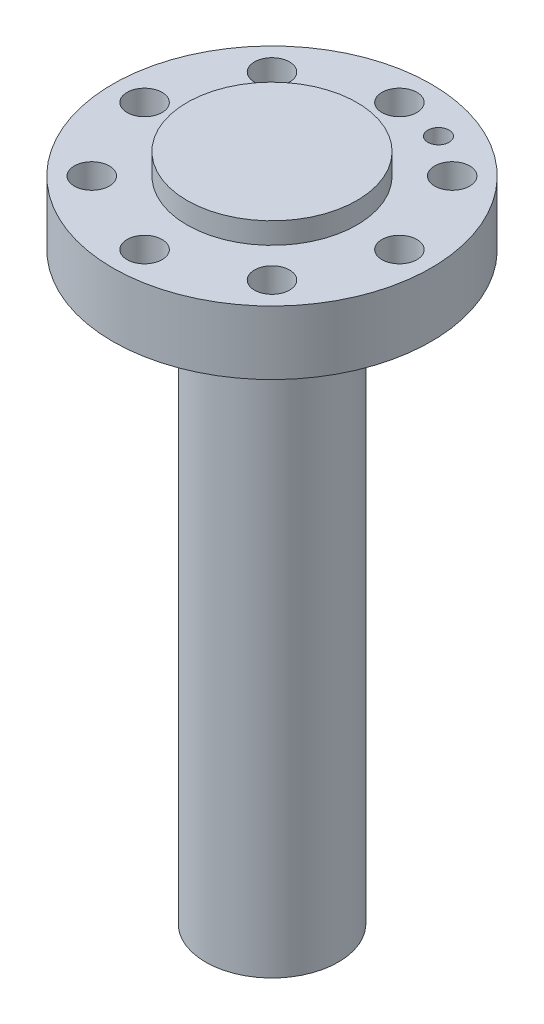
from build123d import *

# Parameters (mm, degrees)
SKETCH_1_R               = 30
EXTRUDE_1_DEPTH          = 122
CUT_EXTRUDE_START        = -12
SKETCH_2_OUTSIDE_W       = 91.722
SKETCH_2_OUTSIDE_H       = 91.722
SKETCH_2_OUTSIDE_R       = 12.5
CUT_EXTRUDE_1_DEPTH      = 118.16655914
HOLE_WIZARD_M6_1_D       = 6.6
SKETCH_7_R               = 16
EXTRUDE_3_DEPTH          = 4
MM_0_D                   = 4
HOLE_WIZARD_M6_1_2_D     = 5
HOLE_WIZARD_M6_1_2_DEPTH = 15
HOLE_WIZARD_M6_1_2_TIP   = 1.502151548


with BuildPart() as part:
    # 草图1 → 凸台-拉伸1 (new body)
    with BuildSketch(Plane(origin=(0, 0, 0), x_dir=(1, 0, 0), z_dir=(0, 1, 0))):
        with Locations(Location((0, 0, 0), (0, 0, 90))):
            Circle(SKETCH_1_R)
    extrude(amount=EXTRUDE_1_DEPTH)

    # 草图2 outside → 切除-拉伸1 (cut, through all)
    with BuildSketch(Plane(origin=(0, 122, 0), x_dir=(1, 0, 0), z_dir=(0, 1, 0)).offset(CUT_EXTRUDE_START)):
        Rectangle(SKETCH_2_OUTSIDE_W, SKETCH_2_OUTSIDE_H)
        with Locations(Location((0, 0, 0), (0, 0, 270))):
            Circle(SKETCH_2_OUTSIDE_R, mode=Mode.SUBTRACT)
    extrude(amount=-CUT_EXTRUDE_1_DEPTH, mode=Mode.SUBTRACT)

    # Hole Wizard M6 _1 (through all)
    with Locations(Plane(origin=(0, 110, 0), x_dir=(-1, 0, 0), z_dir=(0, -1, 0))):
        with Locations((-24, 0), (-16.970562748, 16.970562748), (0, 24), (16.970562748, 16.970562748), (24, 0), (16.970562748, -16.970562748), (0, -24), (-16.970562748, -16.970562748)):
            Hole(HOLE_WIZARD_M6_1_D / 2)

    # 草图7 → 凸台-拉伸3 (add)
    with BuildSketch(Plane(origin=(0, 122, 0), x_dir=(1, 0, 0), z_dir=(0, 1, 0))):
        with Locations(Location((0, 0, 0), (0, 0, 270))):
            Circle(SKETCH_7_R)
    extrude(amount=EXTRUDE_3_DEPTH)

    # 大小mm 暗销孔0 (through all)
    with Locations(Plane(origin=(0, 110, 0), x_dir=(-1, 0, 0), z_dir=(0, -1, 0))):
        with Locations((-9.184402377, 22.17310878)):
            Hole(MM_0_D / 2)

    # Hole Wizard M6 _1 2
    with Locations(Plane(origin=(0, 0, 0), x_dir=(-1, 0, 0), z_dir=(0, -1, 0))):
        with Locations((0, 0)):
            Hole(HOLE_WIZARD_M6_1_2_D / 2, depth=HOLE_WIZARD_M6_1_2_DEPTH)
            with Locations((0, 0, -(HOLE_WIZARD_M6_1_2_DEPTH + HOLE_WIZARD_M6_1_2_TIP / 2))):  # 118° drill point
                Cone(0, HOLE_WIZARD_M6_1_2_D / 2, HOLE_WIZARD_M6_1_2_TIP, mode=Mode.SUBTRACT)


solid = part.part
